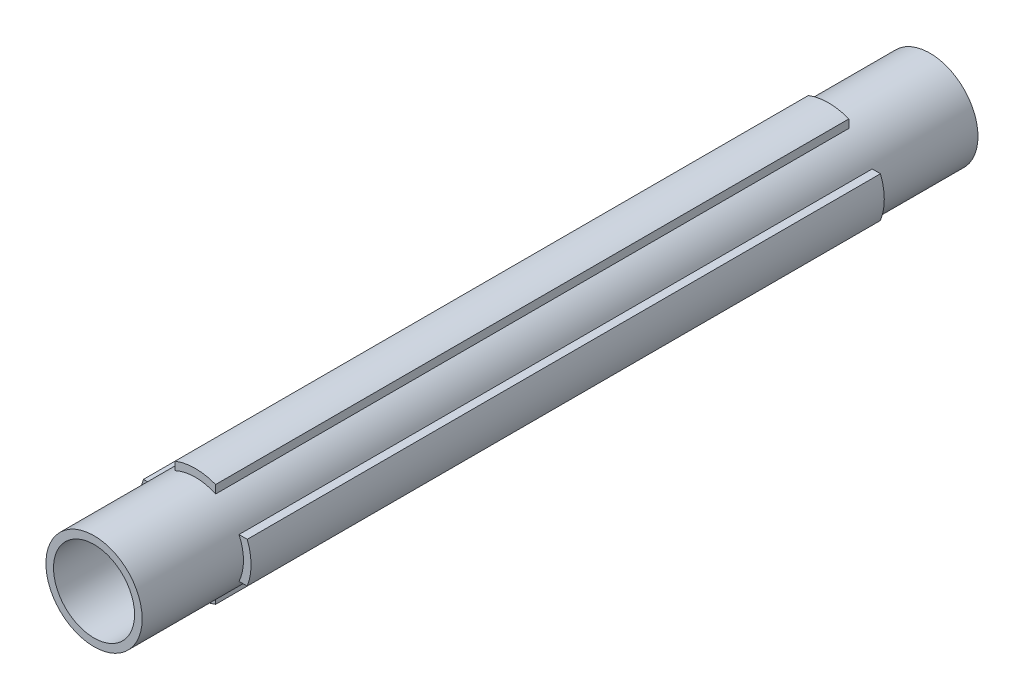
SolidWorks part; units mm, degrees
ref_plane "前视基准面" through (0, 0, 0) normal (0, 0, 1) x (1, 0, 0)
ref_plane "上视基准面" through (0, 0, 0) normal (0, 1, 0) x (1, 0, 0)
ref_plane "右视基准面" through (0, 0, 0) normal (1, 0, 0) x (0, 0, -1)
sketch "草图1" plane through (0, 0, 0) normal (0, 0, 1) x (1, 0, 0)
  line L0 (0, 0) -> (0, 9.5) construction
  line L1 (-2.5, 9.1652) -> (-2.5, 7.5993)
  line L2 (2.5, 9.1652) -> (2.5, 7.5993)
  line L3 (9.1652, 2.5) -> (7.5993, 2.5)
  line L4 (9.1652, -2.5) -> (7.5993, -2.5)
  line L5 (2.5, -9.1652) -> (2.5, -7.5993)
  line L6 (-2.5, -9.1652) -> (-2.5, -7.5993)
  line L7 (-9.1652, -2.5) -> (-7.5993, -2.5)
  line L8 (-9.1652, 2.5) -> (-7.5993, 2.5)
  line L9 (-4, 10.247) -> (-4, 8.6168)
  line L10 (-10.247, 4) -> (-8.6168, 4)
  line L11 (-10.247, -4) -> (-8.6168, -4)
  line L12 (-4, -10.247) -> (-4, -8.6168)
  line L13 (4, -10.247) -> (4, -8.6168)
  line L14 (10.247, -4) -> (8.6168, -4)
  line L15 (10.247, 4) -> (8.6168, 4)
  line L16 (4, 10.247) -> (4, 8.6168)
  arc A0 (-2.5, 7.5993) -> (-7.5993, 2.5) centre (0, 0) ccw
  arc A1 (-9.1652, 2.5) -> (-9.1652, -2.5) centre (0, 0) ccw
  arc A2 (2.5, 9.1652) -> (-2.5, 9.1652) centre (0, 0) ccw
  arc A3 (7.5993, 2.5) -> (2.5, 7.5993) centre (0, 0) ccw
  arc A4 (9.1652, -2.5) -> (9.1652, 2.5) centre (0, 0) ccw
  arc A5 (2.5, -7.5993) -> (7.5993, -2.5) centre (0, 0) ccw
  arc A6 (-2.5, -9.1652) -> (2.5, -9.1652) centre (0, 0) ccw
  arc A7 (-7.5993, -2.5) -> (-2.5, -7.5993) centre (0, 0) ccw
  arc A8 (-4, 8.6168) -> (-8.6168, 4) centre (0, 0) ccw
  arc A9 (-10.247, 4) -> (-10.247, -4) centre (0, 0) ccw
  arc A10 (-8.6168, -4) -> (-4, -8.6168) centre (0, 0) ccw
  arc A11 (-4, -10.247) -> (4, -10.247) centre (0, 0) ccw
  arc A12 (4, -8.6168) -> (8.6168, -4) centre (0, 0) ccw
  arc A13 (10.247, -4) -> (10.247, 4) centre (0, 0) ccw
  arc A14 (8.6168, 4) -> (4, 8.6168) centre (0, 0) ccw
  arc A15 (4, 10.247) -> (-4, 10.247) centre (0, 0) ccw
  dimension "D1" = 16
  dimension "D2" = 19
  dimension "D3" = 2.5
  dimension "D5" = 1.5
  dimension "D4" = 4
extrude "凸台-拉伸1" add sketch "草图1" along normal blind 125
sketch "草图2" plane through (0, 0, 125) normal (0, 0, 1) x (1, 0, 0)
  arc A0 (-2.5, 7.5993) -> (-7.5993, 2.5) centre (0, 0) ccw construction
  arc A1 (-2.5, 7.5993) -> (-7.5993, 2.5) centre (0, 0) ccw construction
  circle A2 centre (0, 0) radius 8
  circle A3 centre (0, 0) radius 9.5
  dimension "D1" = 1.5
extrude "凸台-拉伸2" add sketch "草图2" along normal blind 20 and the other way blind 145
